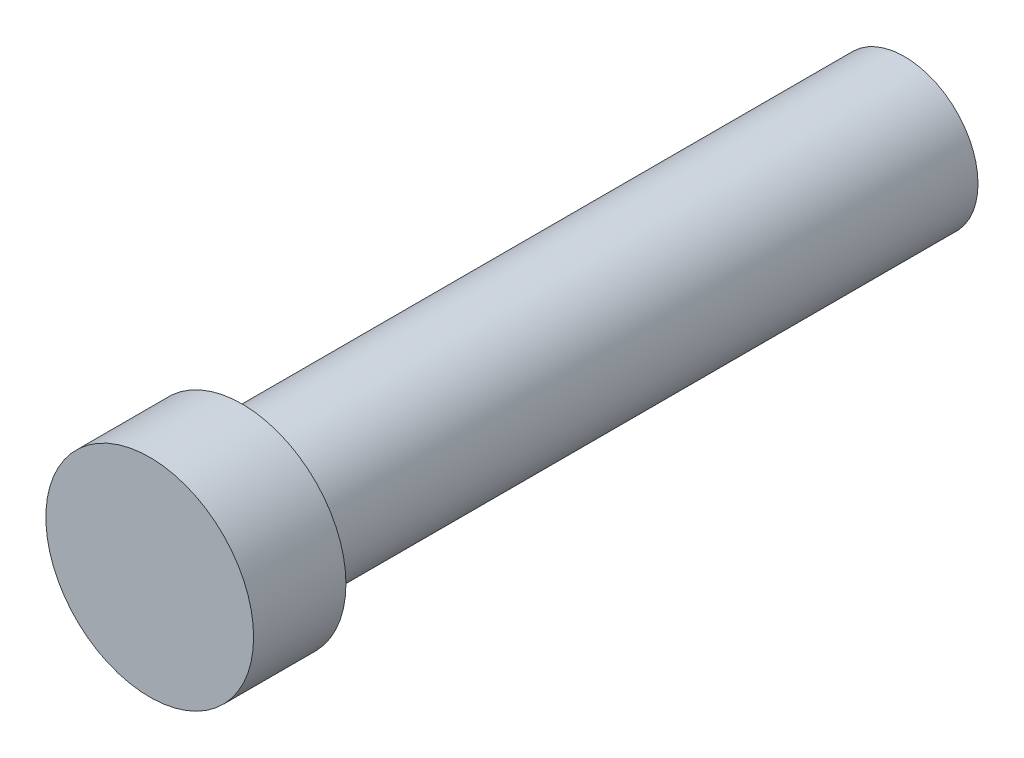
from build123d import *

# Parameters (mm, degrees)
SKETCH_1_R      = 1.59
EXTRUDE_1_DEPTH = 14.35
SKETCH_2_R      = 2.25
EXTRUDE_2_DEPTH = 2


with BuildPart() as part:
    # 草图1 → 凸台-拉伸1 (new body)
    with BuildSketch(Plane.XY):
        Circle(SKETCH_1_R)
    extrude(amount=EXTRUDE_1_DEPTH)


with BuildPart() as body_2:
    # 草图2 → 凸台-拉伸2 (new body)
    with BuildSketch(Plane.XY.offset(14.35)):
        Circle(SKETCH_2_R)
    extrude(amount=EXTRUDE_2_DEPTH)


solid = Compound([part.part, body_2.part])
